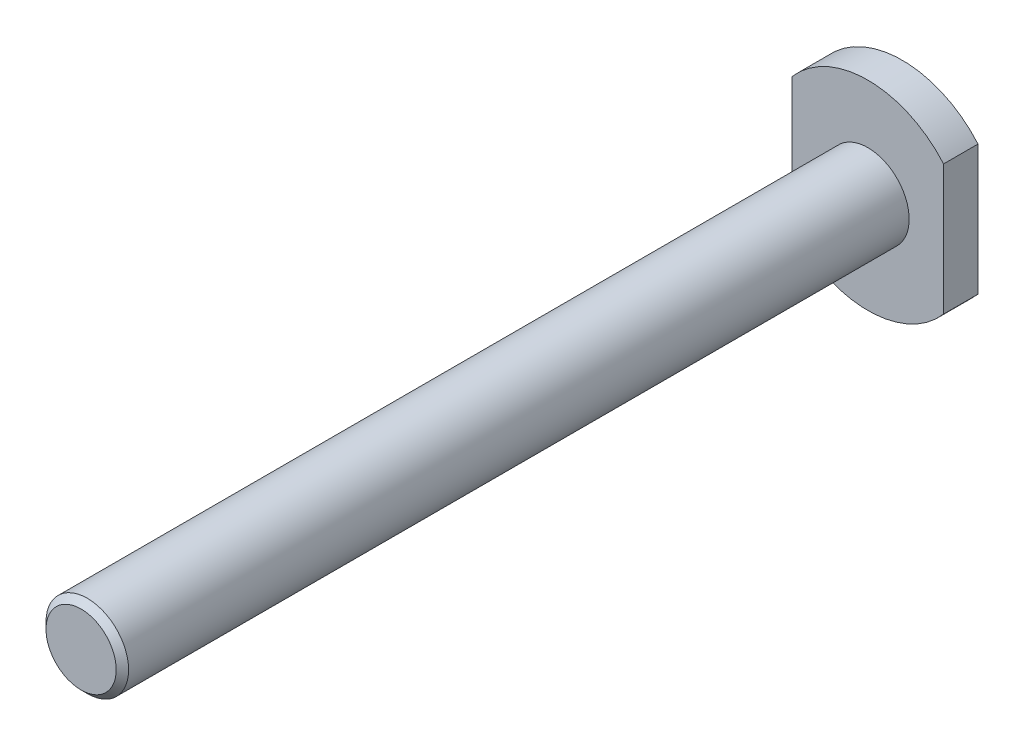
from build123d import *

# Parameters (mm, degrees)
SKETCH1_R           = 6
BOSS_EXTRUDE1_DEPTH = 114.3
CHAMFER2_SIZE       = 0.9
BOSS_EXTRUDE2_DEPTH = 5


with BuildPart() as part:
    # Sketch1 → Boss-Extrude1 (new body)
    with BuildSketch(Plane.XY):
        Circle(SKETCH1_R)
    extrude(amount=BOSS_EXTRUDE1_DEPTH)

    # Chamfer2
    chamfer2_edges = [part.edges().sort_by_distance(p)[0] for p in [
        (-6, 0, 114.3),
    ]]
    chamfer(chamfer2_edges, length=CHAMFER2_SIZE)

    # Sketch2 → Boss-Extrude2 (add)
    with BuildSketch(Plane(origin=(0, 0, 0), x_dir=(-1, 0, 0), z_dir=(0, 0, -1))):
        with BuildLine():
            Line((11, 9.447221814), (11, -9.447221814))
            ThreePointArc((11, -9.447221814), (0, -14.5), (-11, -9.447221814))
            Line((-11, -9.447221814), (-11, 9.447221814))
            ThreePointArc((-11, 9.447221814), (0, 14.5), (11, 9.447221814))
        make_face()
    extrude(amount=BOSS_EXTRUDE2_DEPTH)


solid = part.part
